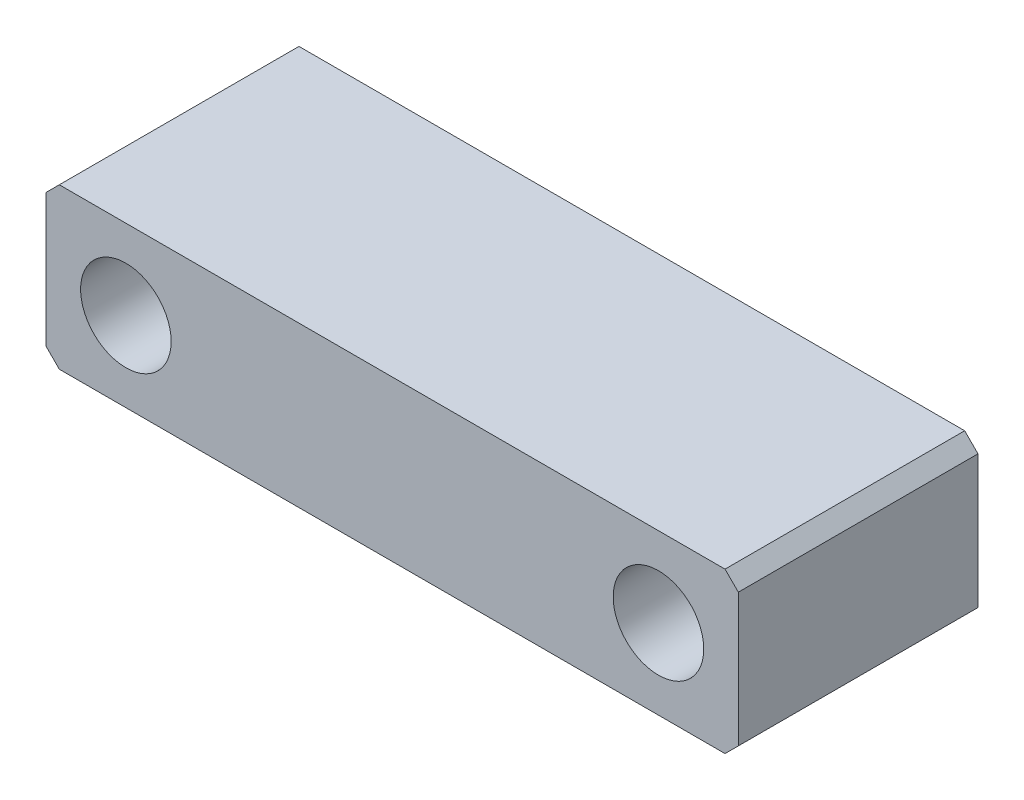
SolidWorks part; units mm, degrees
ref_plane "Front Plane" through (0, 0, 0) normal (0, 0, 1) x (1, 0, 0)
ref_plane "Top Plane" through (0, 0, 0) normal (0, 1, 0) x (1, 0, 0)
ref_plane "Right Plane" through (0, 0, 0) normal (1, 0, 0) x (0, 0, -1)
sketch "Sketch1" plane through (0, 0, 0) normal (0, 0, 1) x (1, 0, 0)
  line L1 (-13, 3) -> (13, 3)
  line L2 (-13, 3) -> (-13, -3)
  line L3 (-13, -3) -> (13, -3)
  line L4 (13, 3) -> (13, -3)
  line L5 (-13, 3) -> (13, -3) construction
  line L6 (-13, -3) -> (13, 3) construction
  point P0 (0, 0)
  dimension "D1" = 6
  dimension "D2" = 26
extrude "Boss-Extrude1" add sketch "Sketch1" along normal blind 9
hole_wizard "M3 Clearance Hole1" positions "Sketch3" profile "Sketch2" hole size "M3" standard "GB"
sketch "Sketch3" plane through (0, 0, 9) normal (0, 0, 1) x (1, 0, 0)
  line L0 (0, 3) -> (0, -3) construction
  line L1 (13, 3) -> (-13, 3) construction
  line L2 (-13, -3) -> (13, -3) construction
  point P1 (-10, 0)
  point P3 (10, 0)
  dimension "D1" = 20
sketch "Sketch2" plane through (-10, 0, 9) normal (1, 0, 0) x (0, -1, 0)
  line L0 (0, 0) -> (0, 31.0215)
  line L1 (0, 31.0215) -> (1.7, 30)
  line L2 (1.7, 30) -> (1.7, 0)
  line L5 (1.7, 0) -> (0, 0)
  line L10 (0, 31.0215) -> (-1.7, 30) construction
  line L11 (0, -6.35) -> (0, 107.95) construction
  dimension "孔直径" = 3.4
  dimension "孔深度" = 30
  dimension "导头角度" = 118
chamfer "Chamfer1" distance 0.5 angle 45 4 edges at (13, 3, 4.5) (13, -3, 4.5) (-13, 3, 4.5) (-13, -3, 4.5)
